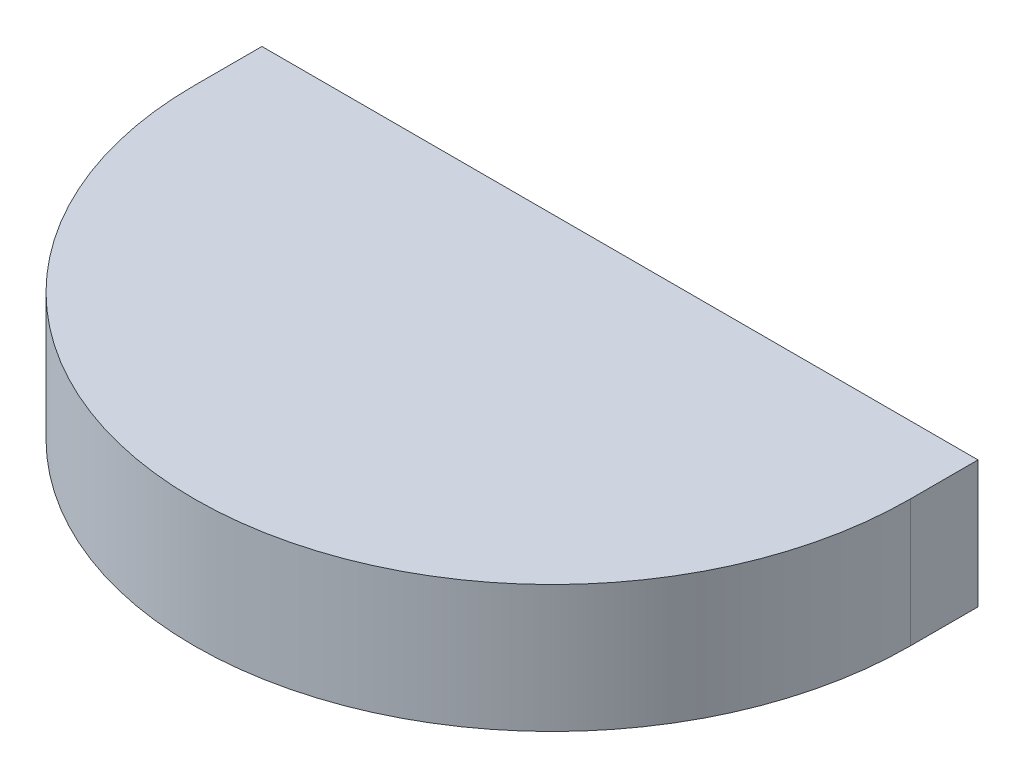
from build123d import *

# Parameters (mm, degrees)
EXTRUDE1_DEPTH = 3.2


with BuildPart() as part:
    # Sketch1 → Extrude1 (new body)
    with BuildSketch(Plane(origin=(0, 0, 0), x_dir=(1, 0, 0), z_dir=(0, 1, 0))):
        with BuildLine():
            Line((-27.128795812, 0), (-27.128795812, 1.7))
            Line((-27.128795812, 1.7), (-9.128795812, 1.7))
            Line((-9.128795812, 1.7), (-9.128795812, 0))
            ThreePointArc((-9.128795812, 0), (-18.128795812, -9), (-27.128795812, 0))
        make_face()
    extrude(amount=EXTRUDE1_DEPTH)


solid = part.part
